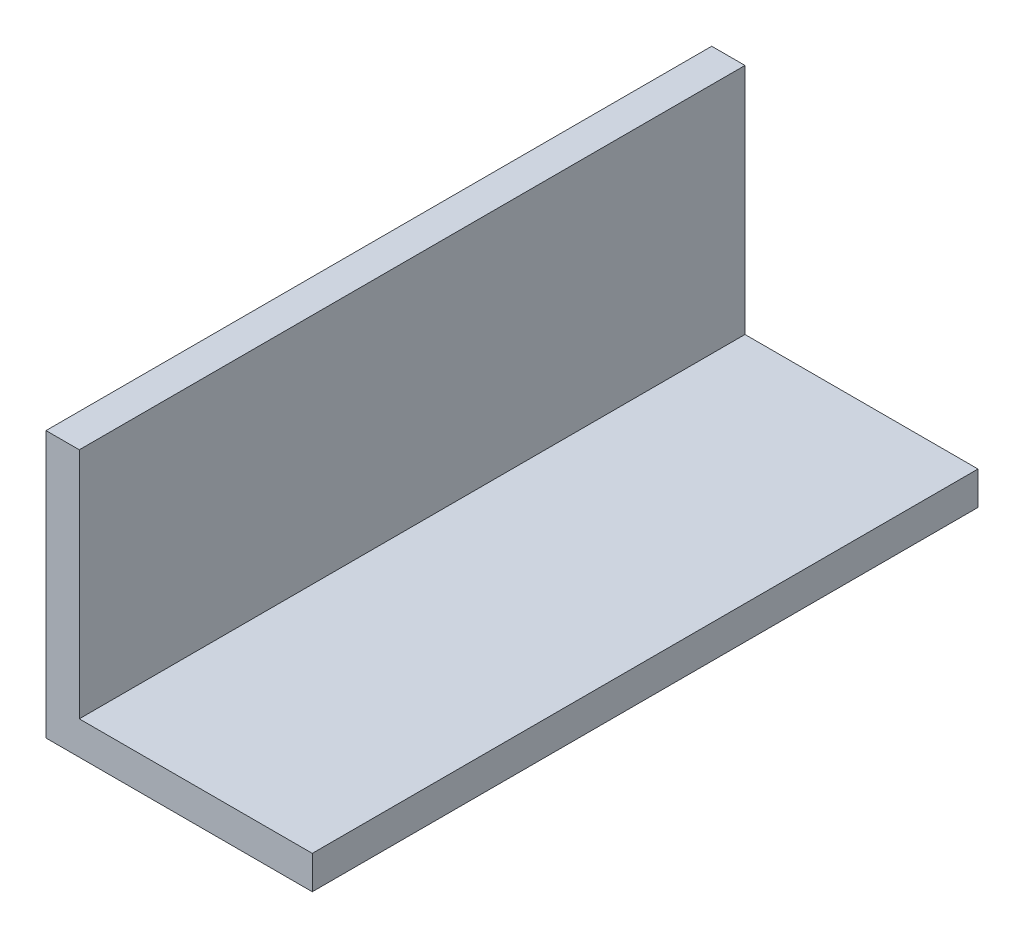
from build123d import *

# Parameters (mm, degrees)
EXTRUDE_1_DEPTH = 100


with BuildPart() as part:
    # 草图1 → 凸台-拉伸1 (new body)
    with BuildSketch(Plane.XY):
        Polygon((0, 0), (0, -40), (40, -40), (40, -35), (5, -35), (5, 0), align=None)
    extrude(amount=EXTRUDE_1_DEPTH)


solid = part.part
